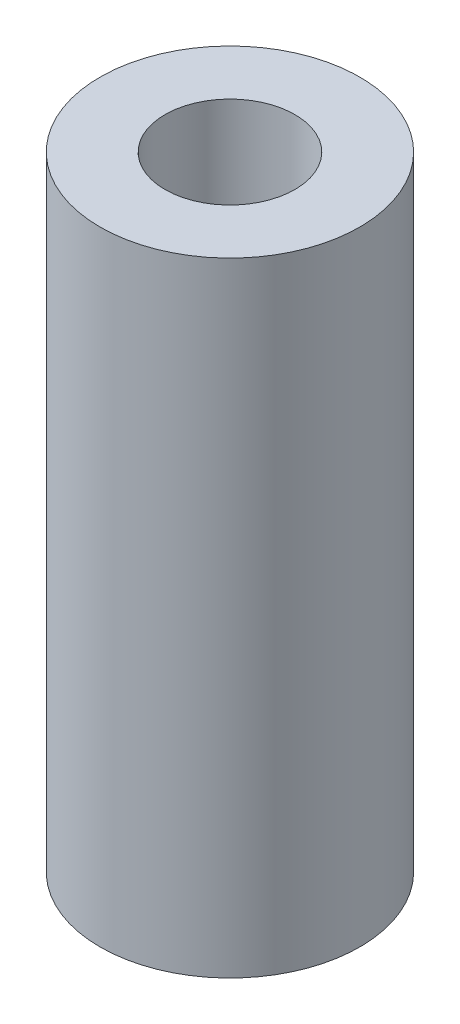
SolidWorks part; units mm, degrees
material "6061 合金"
ref_plane "前视基准面" through (0, 0, 0) normal (0, 0, 1) x (1, 0, 0)
ref_plane "上视基准面" through (0, 0, 0) normal (0, 1, 0) x (1, 0, 0)
ref_plane "右视基准面" through (0, 0, 0) normal (1, 0, 0) x (0, 0, -1)
sketch "草图1" plane through (0, 0, 0) normal (0, 1, 0) x (1, 0, 0)
  circle A0 centre (0, 0) radius 2.5
  dimension "D1" = 5
extrude "凸台-拉伸1" add sketch "草图1" along normal blind 12
sketch "草图2" plane through (0, 12, 0) normal (0, 1, 0) x (1, 0, 0)
  point P0 (0, 0)
hole_wizard "M3 螺纹孔1" positions "草图2" profile "草图3" tap size "M3" standard "GB" end condition through all
sketch "草图3" plane through (0, 12, 0) normal (1, 0, 0) x (0, 0, 1)
  line L0 (0, 0) -> (0, 12)
  line L1 (0, 12) -> (1.25, 12)
  line L2 (1.25, 12) -> (1.25, 0)
  line L5 (1.25, 0) -> (0, 0)
  line L11 (0, -6.35) -> (0, 107.95) construction
  dimension "通孔螺纹孔钻头直径" = 2.5
  dimension "通孔螺纹孔钻头深度" = 12
cosmetic thread "孔螺纹线1" parameters "D2"=3
